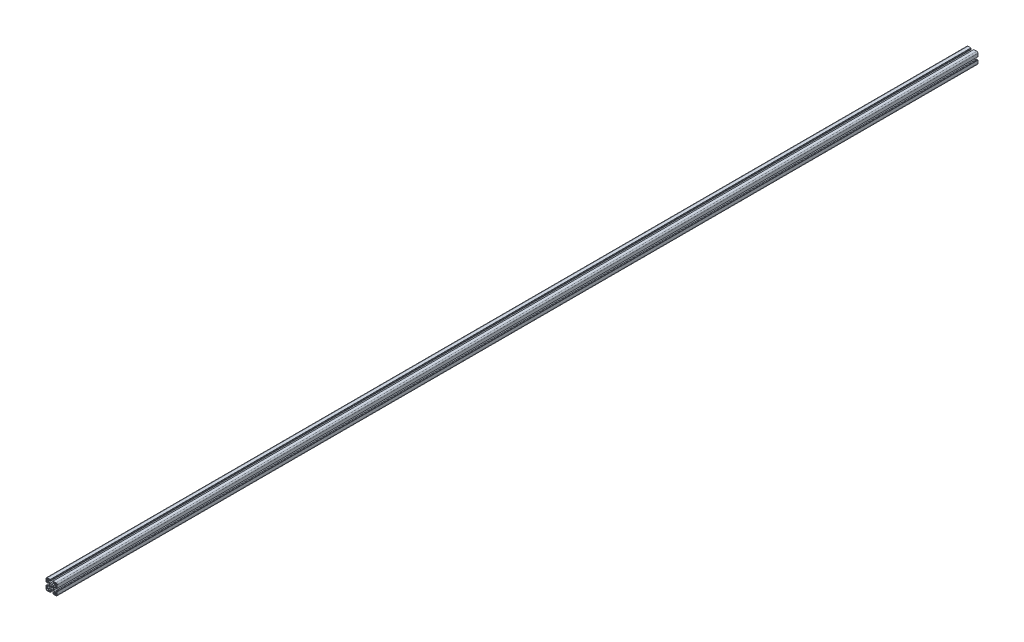
SolidWorks part; units mm, degrees
material "6061 GB/T6892-2006"
ref_plane "前视" through (0, 0, 0) normal (0, 0, 1) x (1, 0, 0)
ref_plane "上视" through (0, 0, 0) normal (0, 1, 0) x (1, 0, 0)
ref_plane "右视" through (0, 0, 0) normal (1, 0, 0) x (0, 0, -1)
sketch "草图1" plane through (0, 0, 0) normal (0, 0, 1) x (1, 0, 0)
  line L0 (-18.9995, -4.1003) -> (-18.9995, -5.1003)
  line L1 (-18.9995, -5.1003) -> (-19.9995, -5.1003)
  line L2 (-19.9995, -5.1003) -> (-19.9995, -15.5003)
  line L3 (-15.4995, -20.0003) -> (-5.0995, -20.0003)
  line L4 (-5.0995, -20.0003) -> (-5.0995, -19.0003)
  line L5 (-5.0995, -19.0003) -> (-4.0995, -19.0003)
  line L6 (-4.0995, -19.0003) -> (-4.0995, -15.5003)
  line L7 (-4.0995, -15.5003) -> (-6.5995, -15.5003)
  line L8 (-6.5995, -15.5003) -> (-6.5995, -16.5003)
  line L9 (-7.5995, -17.5003) -> (-9.7995, -17.5003)
  line L10 (-10.2995, -17.0003) -> (-10.2995, -11.9973)
  line L11 (-10.2995, -11.9973) -> (-5.9025, -7.6003)
  line L12 (-5.9025, -7.6003) -> (-0.5195, -7.6003)
  line L13 (-0.5195, -7.6003) -> (0.0005, -7.3003)
  line L14 (0.0005, -7.3003) -> (0.5195, -7.6003)
  line L15 (0.5195, -7.6003) -> (5.9035, -7.6003)
  line L16 (5.9035, -7.6003) -> (10.3005, -11.9973)
  line L17 (10.3005, -11.9973) -> (10.3005, -17.0003)
  line L18 (9.8005, -17.5003) -> (7.6005, -17.5003)
  line L19 (6.6005, -16.5003) -> (6.6005, -15.5003)
  line L20 (6.6005, -15.5003) -> (4.1005, -15.5003)
  line L21 (4.1005, -15.5003) -> (4.1005, -19.0003)
  line L22 (4.1005, -19.0003) -> (5.1005, -19.0003)
  line L23 (5.1005, -19.0003) -> (5.1005, -20.0003)
  line L24 (5.1005, -20.0003) -> (15.5005, -20.0003)
  line L25 (20.0005, -15.5003) -> (20.0005, -5.1003)
  line L26 (20.0005, -5.1003) -> (19.0005, -5.1003)
  line L27 (19.0005, -5.1003) -> (19.0005, -4.1003)
  line L28 (19.0005, -4.1003) -> (15.5005, -4.1003)
  line L29 (15.5005, -4.1003) -> (15.5005, -6.6003)
  line L30 (15.5005, -6.6003) -> (16.5005, -6.6003)
  line L31 (17.5005, -7.6003) -> (17.5005, -9.8003)
  line L32 (17.0005, -10.3003) -> (11.9975, -10.3003)
  line L33 (11.9975, -10.3003) -> (7.6005, -5.9033)
  line L34 (7.6005, -5.9033) -> (7.6005, -0.5203)
  line L35 (7.6005, -0.5203) -> (7.3005, -0.0003)
  line L36 (7.3005, -0.0003) -> (7.6005, 0.5197)
  line L37 (7.6005, 0.5197) -> (7.6005, 5.9027)
  line L38 (7.6005, 5.9027) -> (11.9975, 10.2997)
  line L39 (11.9975, 10.2997) -> (17.0005, 10.2997)
  line L40 (17.5005, 9.7997) -> (17.5005, 7.5997)
  line L41 (16.5005, 6.5997) -> (15.5005, 6.5997)
  line L42 (15.5005, 6.5997) -> (15.5005, 4.0997)
  line L43 (15.5005, 4.0997) -> (19.0005, 4.0997)
  line L44 (19.0005, 4.0997) -> (19.0005, 5.0997)
  line L45 (19.0005, 5.0997) -> (20.0005, 5.0997)
  line L46 (20.0005, 5.0997) -> (20.0005, 15.4997)
  line L47 (15.5005, 19.9997) -> (5.1005, 19.9997)
  line L48 (5.1005, 19.9997) -> (5.1005, 18.9997)
  line L49 (5.1005, 18.9997) -> (4.1005, 18.9997)
  line L50 (4.1005, 18.9997) -> (4.1005, 15.4997)
  line L51 (4.1005, 15.4997) -> (6.6005, 15.4997)
  line L52 (7.6005, 17.4997) -> (9.8005, 17.4997)
  line L53 (10.3005, 16.9997) -> (10.3005, 11.9967)
  line L54 (10.3005, 11.9967) -> (5.9035, 7.5997)
  line L55 (5.9035, 7.5997) -> (0.5195, 7.5997)
  line L56 (0.5195, 7.5997) -> (0.0005, 7.2997)
  line L57 (0.0005, 7.2997) -> (-0.5195, 7.5997)
  line L58 (-0.5195, 7.5997) -> (-5.9025, 7.5997)
  line L59 (-5.9025, 7.5997) -> (-10.2995, 11.9967)
  line L60 (-10.2995, 11.9967) -> (-10.2995, 16.9997)
  line L61 (-9.7995, 17.4997) -> (-7.5995, 17.4997)
  line L62 (-6.5995, 16.4997) -> (-6.5995, 15.4997)
  line L63 (-6.5995, 15.4997) -> (-4.0995, 15.4997)
  line L64 (-4.0995, 15.4997) -> (-4.0995, 18.9997)
  line L65 (-4.0995, 18.9997) -> (-5.0995, 18.9997)
  line L66 (-5.0995, 18.9997) -> (-5.0995, 19.9997)
  line L67 (-5.0995, 19.9997) -> (-15.4995, 19.9997)
  line L68 (-19.9995, 15.4997) -> (-19.9995, 5.0997)
  line L69 (-19.9995, 5.0997) -> (-18.9995, 5.0997)
  line L70 (-18.9995, 5.0997) -> (-18.9995, 4.0997)
  line L71 (-18.9995, 4.0997) -> (-15.4995, 4.0997)
  line L72 (-15.4995, 4.0997) -> (-15.4995, 6.5997)
  line L73 (-15.4995, 6.5997) -> (-16.4995, 6.5997)
  line L74 (-17.4995, 7.5997) -> (-17.4995, 9.7997)
  line L75 (-16.9995, 10.2997) -> (-11.9965, 10.2997)
  line L76 (-11.9965, 10.2997) -> (-7.5995, 5.9027)
  line L77 (-7.5995, 5.9027) -> (-7.5995, 0.5197)
  line L78 (-7.5995, 0.5197) -> (-7.2995, -0.0003)
  line L79 (-7.2995, -0.0003) -> (-7.5995, -0.5203)
  line L80 (-7.5995, -0.5203) -> (-7.5995, -5.9033)
  line L81 (-7.5995, -5.9033) -> (-11.9965, -10.3003)
  line L82 (-11.9965, -10.3003) -> (-16.9995, -10.3003)
  line L83 (-17.4995, -9.8003) -> (-17.4995, -7.6003)
  line L84 (-16.4995, -6.6003) -> (-15.4995, -6.6003)
  line L85 (-15.4995, -6.6003) -> (-15.4995, -4.1003)
  line L86 (-15.4995, -4.1003) -> (-18.9995, -4.1003)
  line L87 (15.5005, -18.0003) -> (11.8005, -18.0003)
  line L88 (11.8005, -18.0003) -> (11.8005, -11.8003)
  line L89 (11.8005, -11.8003) -> (18.0005, -11.8003)
  line L90 (18.0005, -11.8003) -> (18.0005, -15.5003)
  line L91 (18.0005, 11.7997) -> (11.8005, 11.7997)
  line L92 (11.8005, 11.7997) -> (11.8005, 17.9997)
  line L93 (11.8005, 17.9997) -> (15.5005, 17.9997)
  line L94 (18.0005, 15.4997) -> (18.0005, 11.7997)
  line L95 (-1.8145, -2.8753) -> (-3.0044, -4.0665)
  line L96 (-3.0044, -4.0665) -> (-4.0656, -3.0052)
  line L97 (-4.0656, -3.0052) -> (-2.8745, -1.8153)
  line L98 (-2.8745, 1.8147) -> (-4.0644, 3.0058)
  line L99 (-4.0644, 3.0058) -> (-3.0044, 4.0658)
  line L100 (-3.0044, 4.0658) -> (-1.8145, 2.8747)
  line L101 (1.8145, 2.8747) -> (3.0055, 4.0657)
  line L102 (3.0055, 4.0657) -> (4.0666, 3.0045)
  line L103 (4.0666, 3.0045) -> (2.8755, 1.8147)
  line L104 (2.8755, -1.8153) -> (4.0666, -3.0052)
  line L105 (4.0666, -3.0052) -> (3.0055, -4.0663)
  line L106 (3.0055, -4.0663) -> (1.8145, -2.8753)
  line L107 (-17.9995, -15.5003) -> (-17.9995, -11.8003)
  line L108 (-17.9995, -11.8003) -> (-11.7995, -11.8003)
  line L109 (-11.7995, -11.8003) -> (-11.7995, -18.0003)
  line L110 (-11.7995, -18.0003) -> (-15.4995, -18.0003)
  line L111 (-11.7995, 17.9997) -> (-11.7995, 11.7997)
  line L112 (-11.7995, 11.7997) -> (-17.9995, 11.7997)
  line L113 (-17.9995, 11.7997) -> (-17.9995, 15.4997)
  line L114 (-15.4995, 17.9997) -> (-11.7995, 17.9997)
  arc A0 (-19.9995, -15.5003) -> (-15.4995, -20.0003) centre (-15.4995, -15.5003) ccw
  arc A1 (-6.5995, -16.5003) -> (-7.5995, -17.5003) centre (-7.5995, -16.5003) cw
  arc A2 (-9.7995, -17.5003) -> (-10.2995, -17.0003) centre (-9.7995, -17.0003) cw
  arc A3 (10.3005, -17.0003) -> (9.8005, -17.5003) centre (9.8005, -17.0003) cw
  arc A4 (7.6005, -17.5003) -> (6.6005, -16.5003) centre (7.6005, -16.5003) cw
  arc A5 (15.5005, -20.0003) -> (20.0005, -15.5003) centre (15.5005, -15.5003) ccw
  arc A6 (16.5005, -6.6003) -> (17.5005, -7.6003) centre (16.5005, -7.6003) cw
  arc A7 (17.5005, -9.8003) -> (17.0005, -10.3003) centre (17.0005, -9.8003) cw
  arc A8 (17.0005, 10.2997) -> (17.5005, 9.7997) centre (17.0005, 9.7997) cw
  arc A9 (17.5005, 7.5997) -> (16.5005, 6.5997) centre (16.5005, 7.5997) cw
  arc A10 (20.0005, 15.4997) -> (15.5005, 19.9997) centre (15.5005, 15.4997) ccw
  arc A11 (6.6005, 15.4997) -> (6.6005, 16.4997) centre (7.1003, 15.9997) cw
  arc A12 (6.6005, 16.4997) -> (7.6005, 17.4997) centre (7.6005, 16.4997) cw
  arc A13 (9.8005, 17.4997) -> (10.3005, 16.9997) centre (9.8005, 16.9997) cw
  arc A14 (-10.2995, 16.9997) -> (-9.7995, 17.4997) centre (-9.7995, 16.9997) cw
  arc A15 (-7.5995, 17.4997) -> (-6.5995, 16.4997) centre (-7.5995, 16.4997) cw
  arc A16 (-15.4995, 19.9997) -> (-19.9995, 15.4997) centre (-15.4995, 15.4997) ccw
  arc A17 (-16.4995, 6.5997) -> (-17.4995, 7.5997) centre (-16.4995, 7.5997) cw
  arc A18 (-17.4995, 9.7997) -> (-16.9995, 10.2997) centre (-16.9995, 9.7997) cw
  arc A19 (-16.9995, -10.3003) -> (-17.4995, -9.8003) centre (-16.9995, -9.8003) cw
  arc A20 (-17.4995, -7.6003) -> (-16.4995, -6.6003) centre (-16.4995, -7.6003) cw
  arc A21 (18.0005, -15.5003) -> (15.5005, -18.0003) centre (15.5005, -15.5003) cw
  arc A22 (15.5005, 17.9997) -> (18.0005, 15.4997) centre (15.5005, 15.4997) cw
  arc A23 (-2.8745, -1.8153) -> (-2.8745, 1.8147) centre (0.0005, -0.0003) cw
  arc A24 (-1.8145, 2.8747) -> (1.8145, 2.8747) centre (0, -0.0007) cw
  arc A25 (2.8755, 1.8147) -> (2.8755, -1.8153) centre (0.0005, -0.0003) cw
  arc A26 (1.8145, -2.8753) -> (-1.8145, -2.8753) centre (0, 0) cw
  arc A27 (-15.4995, -18.0003) -> (-17.9995, -15.5003) centre (-15.4995, -15.5003) cw
  arc A28 (-17.9995, 15.4997) -> (-15.4995, 17.9997) centre (-15.4995, 15.4997) cw
extrude "凸台-拉伸1" add sketch "草图1" against normal blind 3280
hole_wizard "打孔尺寸(%根据)内六角圆柱头螺钉的类型2" positions "草图2" profile "草图3" counterbore size "M6" standard "GB" end condition through all
sketch "草图2" plane through (0.0008, -20.0003, 0) normal (0, 1, 0) x (0, 0, 1)
  line L13 (-3280, 19.9997) -> (0, 19.9997) construction
  line L17 (0, 15.4997) -> (0, 5.0997) construction
  point P0 (-80, -0.0003)
  point P2 (-1080, -0.0003)
  point P20 (-2200, -0.0003)
  point P24 (-3200, -0.0003)
  dimension "D1" = 1000
  dimension "D2" = 80
  dimension "D3" = 20
  dimension "D4" = 20
  dimension "D5" = 1000
  dimension "D6" = 80
sketch "草图3" plane through (0.0005, -20.0003, -80) normal (1, 0, 0) x (0, 0, -1)
  line L0 (0, 0) -> (0, 40)
  line L1 (0, 40) -> (3.3, 40)
  line L3 (3.3, 40) -> (3.3, 6.8)
  line L4 (3.3, 6.8) -> (5.5, 6.8)
  line L5 (5.5, 6.8) -> (5.5, 0)
  line L7 (5.5, 0) -> (0, 0)
  line L11 (0, -6.35) -> (0, 107.95) construction
  dimension "通孔孔直径" = 6.6
  dimension "通孔孔深度" = 40
  dimension "柱形沉头孔直径" = 11
  dimension "柱形沉头孔深度" = 6.8
hole_wizard "打孔尺寸(%根据)内六角圆柱头螺钉的类型2" positions "草图4" profile "草图5" counterbore size "M6" standard "GB" end condition through all
sketch "草图4" plane through (0, 19.9997, 0) normal (0, 1, 0) x (1, 0, 0)
  line L15 (20.0005, 3280) -> (20.0005, 0) construction
  point P0 (0.0005, 1080)
  point P3 (0.0005, 1640)
  point P7 (0.0005, 2200)
  point P10 (0.0005, 3200)
  point P94 (0.0005, 80)
  point P103 (1.0946, 77.8588)
  point P108 (20.0005, 1082.0263)
  dimension "D1" = 80
  dimension "D3" = 20
  dimension "D5" = 1000
  dimension "D6" = 20
sketch "草图5" plane through (0.0005, 19.9997, -1080) normal (1, 0, 0) x (0, 0, 1)
  line L0 (0, 0) -> (0, 40)
  line L1 (0, 40) -> (3.3, 40)
  line L3 (3.3, 40) -> (3.3, 6.8)
  line L4 (3.3, 6.8) -> (5.5, 6.8)
  line L5 (5.5, 6.8) -> (5.5, 0)
  line L7 (5.5, 0) -> (0, 0)
  line L11 (0, -6.35) -> (0, 107.95) construction
  dimension "通孔孔直径" = 6.6
  dimension "通孔孔深度" = 40
  dimension "柱形沉头孔直径" = 11
  dimension "柱形沉头孔深度" = 6.8
